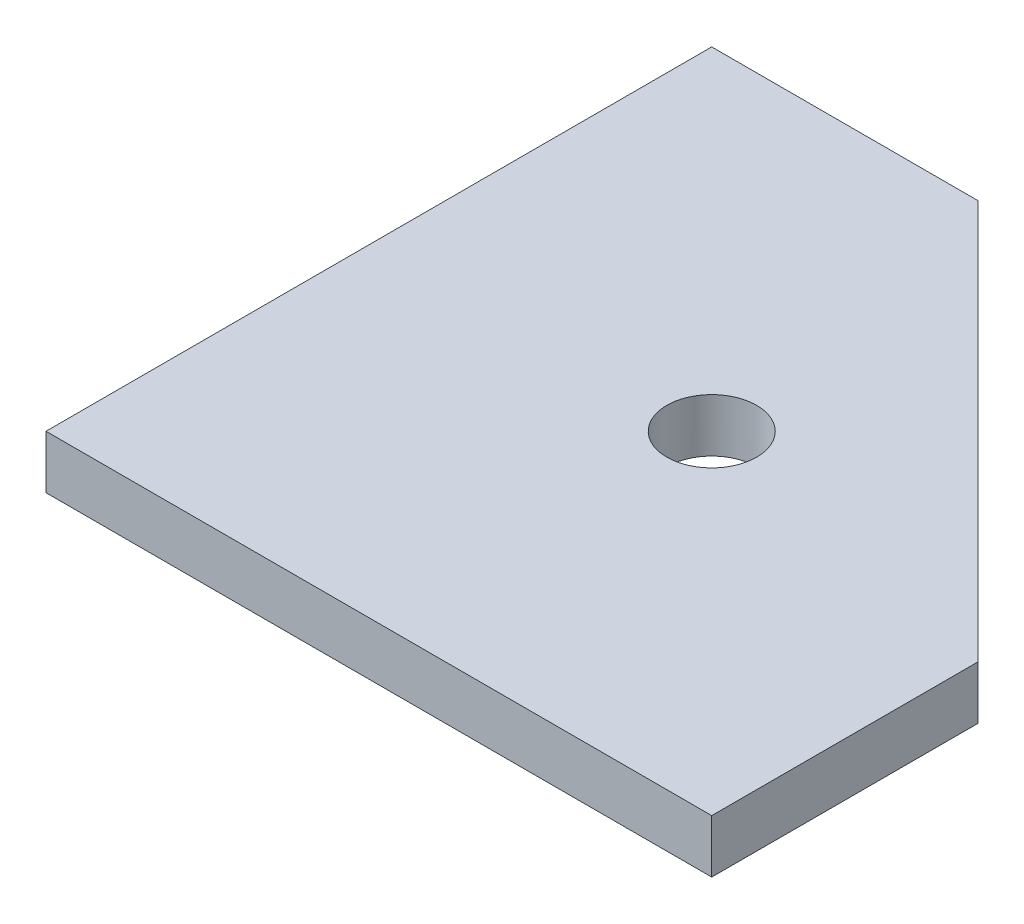
from build123d import *

# Parameters (mm, degrees)
BOSS_EXTRUDE1_DEPTH       = 8
M12_CLEARANCE_HOLE1_D     = 13.5
M12_CLEARANCE_HOLE1_DEPTH = 60
M12_CLEARANCE_HOLE1_TIP   = 4.055809178


with BuildPart() as part:
    # Sketch1 → Boss-Extrude1 (new body)
    with BuildSketch(Plane(origin=(0, 0, 0), x_dir=(1, 0, 0), z_dir=(0, 1, 0))):
        Polygon((0, 0), (100, 0), (100, 40), (40, 100), (0, 100), align=None)
    extrude(amount=BOSS_EXTRUDE1_DEPTH)

    # M12 Clearance Hole1
    with Locations(Plane(origin=(0, 8, 0), x_dir=(1, 0, 0), z_dir=(0, 1, 0))):
        with Locations((50, 50)):
            Hole(M12_CLEARANCE_HOLE1_D / 2, depth=M12_CLEARANCE_HOLE1_DEPTH)
            with Locations((0, 0, -(M12_CLEARANCE_HOLE1_DEPTH + M12_CLEARANCE_HOLE1_TIP / 2))):  # 118° drill point
                Cone(0, M12_CLEARANCE_HOLE1_D / 2, M12_CLEARANCE_HOLE1_TIP, mode=Mode.SUBTRACT)


solid = part.part
